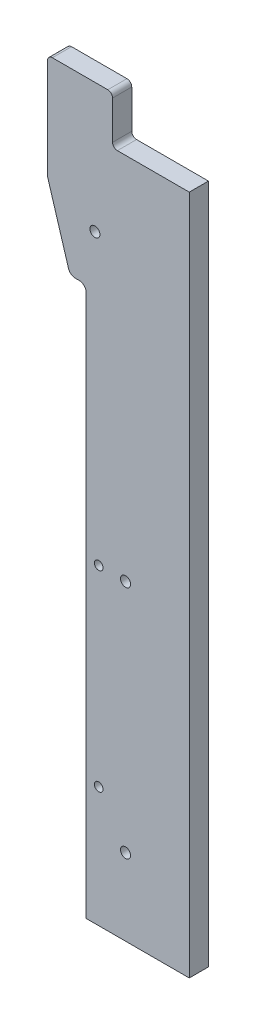
from build123d import *

# Parameters (mm, degrees)
SKETCH1_R           = 9
BOSS_EXTRUDE1_DEPTH = 40
M24_TAPPED_HOLE1_D  = 21
FILLET1_R           = 15
FILLET2_R           = 10


with BuildPart() as part:
    # Sketch1 → Boss-Extrude1 (new body)
    with BuildSketch(Plane.XY):
        Polygon((0, 0), (0, 1145.516137583), (-33.72387302, 1145.516137583), (-80.68, 1300), (-80.68, 1520), (55, 1520), (55, 1420), (215, 1420), (215, 0), align=None)
        with Locations((26, 251)):
            Circle(SKETCH1_R, mode=Mode.SUBTRACT)
        with Locations((26, 651)):
            Circle(SKETCH1_R, mode=Mode.SUBTRACT)
    extrude(amount=BOSS_EXTRUDE1_DEPTH)

    # M24 Tapped Hole1 (through all)
    with Locations(Plane(origin=(18.132788177, 1250, 0), x_dir=(-1, 0, 0), z_dir=(0, 0, -1))):
        with Locations((0, 0), (-63.867211823, -600), (-63.867211823, -1090)):
            Hole(M24_TAPPED_HOLE1_D / 2)

    # Fillet1
    fillet1_edges = [part.edges().sort_by_distance(p)[0] for p in [
        (0, 1145.516137583, 20),
        (-33.72387302, 1145.516137583, 20),
    ]]
    fillet(fillet1_edges, radius=FILLET1_R)

    # Fillet2
    fillet2_edges = [part.edges().sort_by_distance(p)[0] for p in [
        (-80.68, 1520, 20),
        (55, 1520, 20),
        (55, 1420, 20),
    ]]
    fillet(fillet2_edges, radius=FILLET2_R)


solid = part.part
